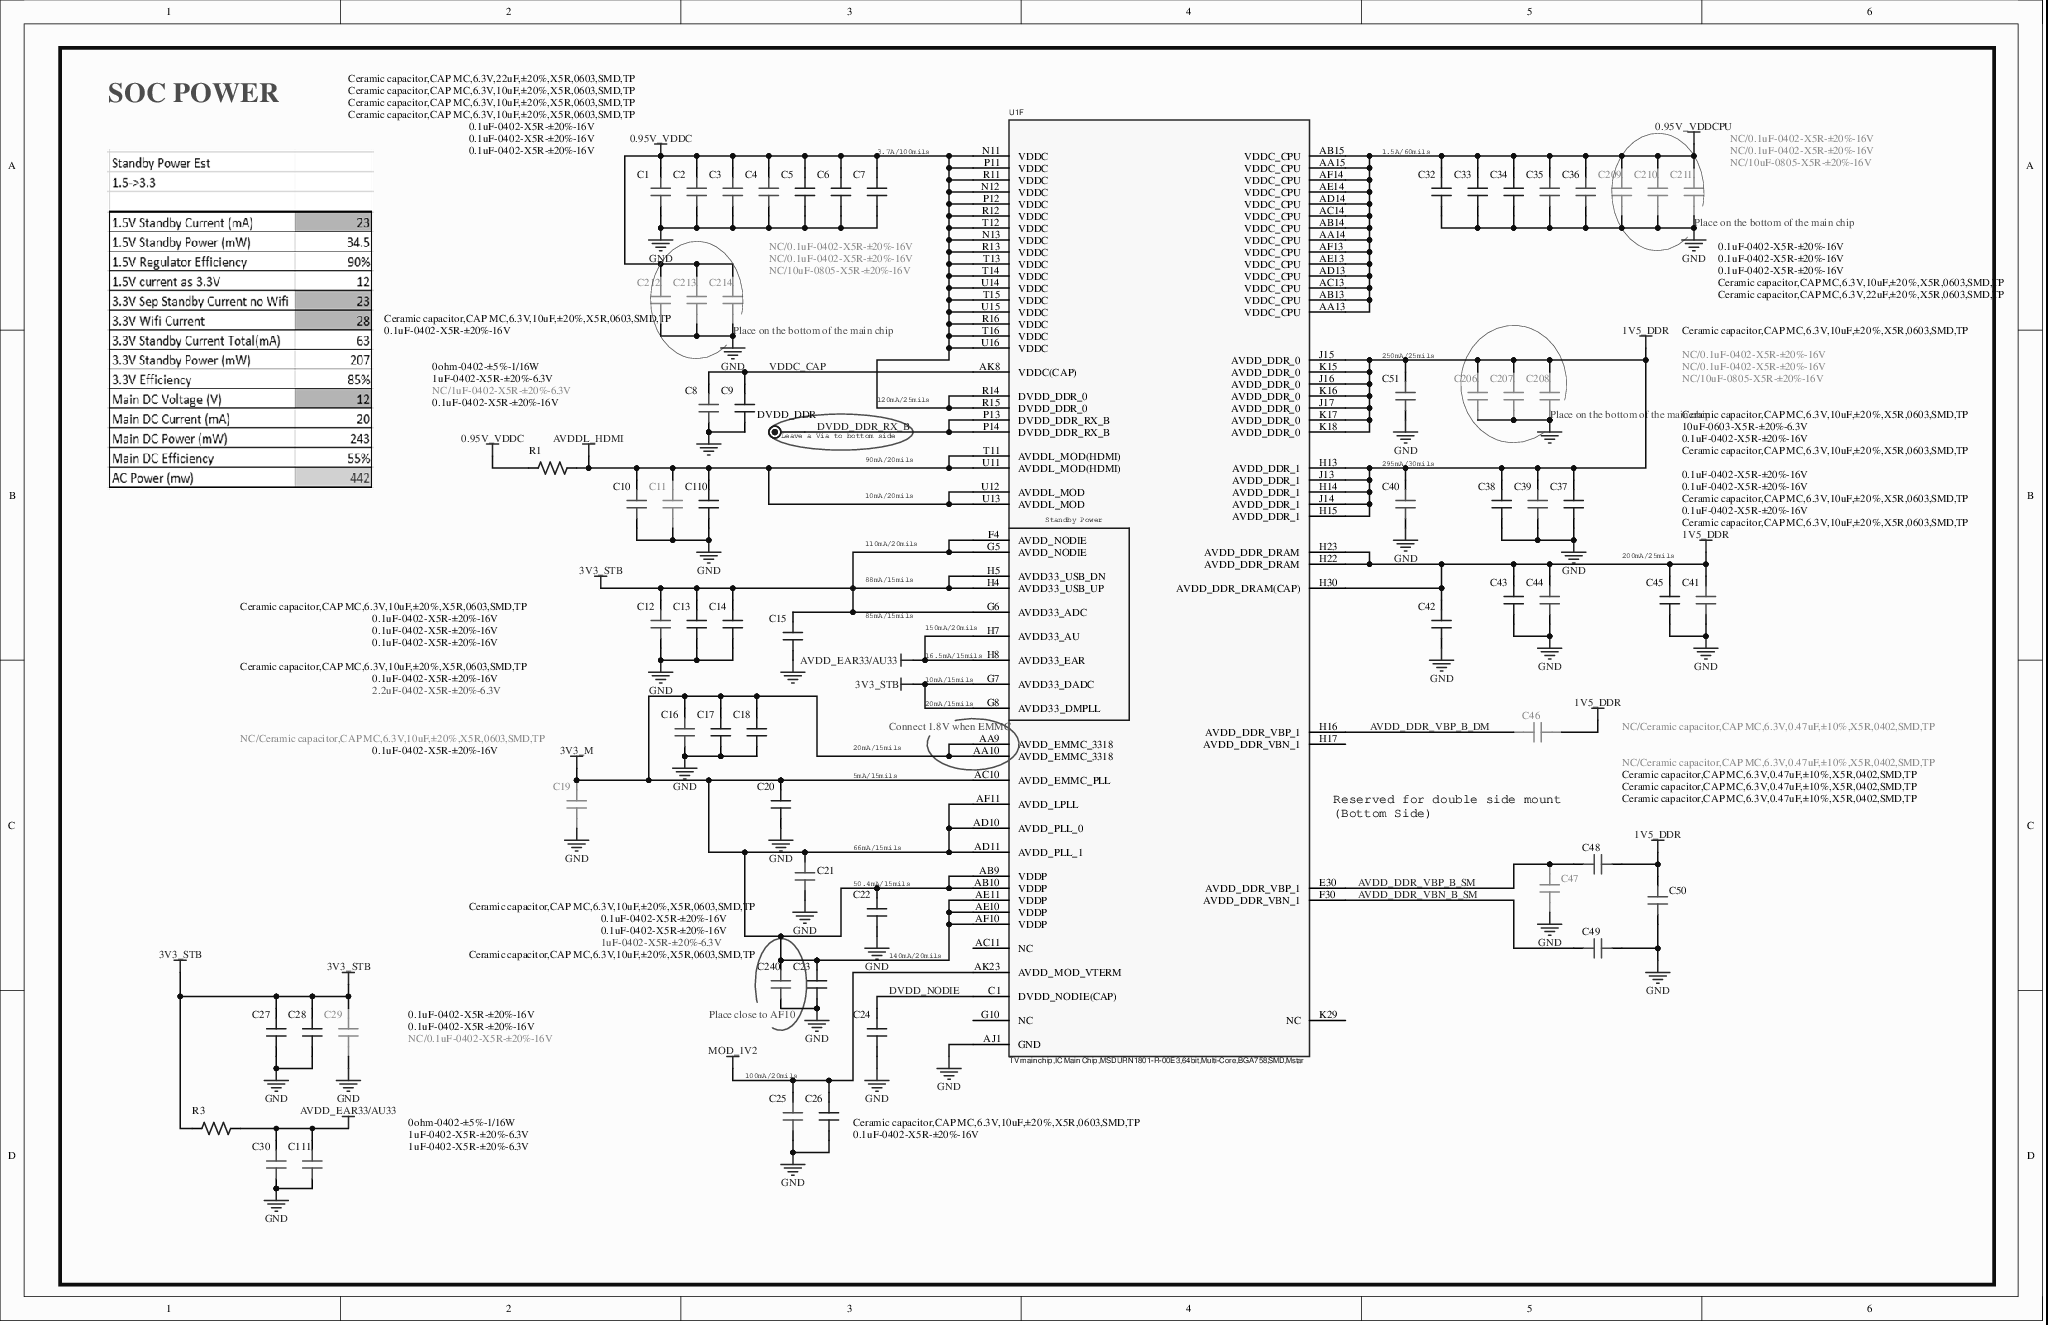
[diagram p0: MISC86290-7.SchDoc]
# Altium project MISC86290.PrjPcb (part 6 of 13)

## Sheet MISC86290-7.SchDoc
size 431 x 279 mm

### Parts
C1  Ceramic capacitor,CAP MC,6.3V,22uF,±20%,X5R,0603,SMD,TP  [C0603]
C2  Ceramic capacitor,CAP MC,6.3V,10uF,±20%,X5R,0603,SMD,TP  [C0603]
C3  Ceramic capacitor,CAP MC,6.3V,10uF,±20%,X5R,0603,SMD,TP  [C0603]
C4  Ceramic capacitor,CAP MC,6.3V,10uF,±20%,X5R,0603,SMD,TP  [C0603]
C5  0.1uF-0402-X5R-±20%-16V  [C0402]
C6  0.1uF-0402-X5R-±20%-16V  [C0402]
C7  0.1uF-0402-X5R-±20%-16V  [C0402]
C8  Ceramic capacitor,CAP MC,6.3V,10uF,±20%,X5R,0603,SMD,TP  [C0603]
C9  0.1uF-0402-X5R-±20%-16V  [C0402]
C10  1uF-0402-X5R-±20%-6.3V  [C0402]
C11  NC/1uF-0402-X5R-±20%-6.3V  [C0402]
C12  Ceramic capacitor,CAP MC,6.3V,10uF,±20%,X5R,0603,SMD,TP  [C0603]
C13  0.1uF-0402-X5R-±20%-16V  [C0402]
C14  0.1uF-0402-X5R-±20%-16V  [C0402]
C15  0.1uF-0402-X5R-±20%-16V  [C0402]
C16  Ceramic capacitor,CAP MC,6.3V,10uF,±20%,X5R,0603,SMD,TP  [C0603]
C17  0.1uF-0402-X5R-±20%-16V  [C0402]
C18  2.2uF-0402-X5R-±20%-6.3V  [C0402]
C19  NC/Ceramic capacitor,CAP MC,6.3V,10uF,±20%,X5R,0603,SMD,TP  [C0603]
C20  0.1uF-0402-X5R-±20%-16V  [C0402]
C21  Ceramic capacitor,CAP MC,6.3V,10uF,±20%,X5R,0603,SMD,TP  [C0603]
C22  0.1uF-0402-X5R-±20%-16V  [C0402]
C23  0.1uF-0402-X5R-±20%-16V  [C0402]
C24  1uF-0402-X5R-±20%-6.3V  [C0402]
C25  Ceramic capacitor,CAP MC,6.3V,10uF,±20%,X5R,0603,SMD,TP  [C0603]
C26  0.1uF-0402-X5R-±20%-16V  [C0402]
C27  0.1uF-0402-X5R-±20%-16V  [C0402]
C28  0.1uF-0402-X5R-±20%-16V  [C0402]
C29  NC/0.1uF-0402-X5R-±20%-16V  [C0402]
C30  1uF-0402-X5R-±20%-6.3V  [C0402]
C32  0.1uF-0402-X5R-±20%-16V  [C0402]
C33  0.1uF-0402-X5R-±20%-16V  [C0402]
C34  0.1uF-0402-X5R-±20%-16V  [C0402]
C35  Ceramic capacitor,CAP MC,6.3V,10uF,±20%,X5R,0603,SMD,TP  [C0603]
C36  Ceramic capacitor,CAP MC,6.3V,22uF,±20%,X5R,0603,SMD,TP  [C0603]
C37  10uF-0603-X5R-±20%-6.3V  [C0603]
C38  0.1uF-0402-X5R-±20%-16V  [C0402]
C39  Ceramic capacitor,CAP MC,6.3V,10uF,±20%,X5R,0603,SMD,TP  [C0603]
C40  Ceramic capacitor,CAP MC,6.3V,10uF,±20%,X5R,0603,SMD,TP  [C0603]
C41  Ceramic capacitor,CAP MC,6.3V,10uF,±20%,X5R,0603,SMD,TP  [C0603]
C42  0.1uF-0402-X5R-±20%-16V  [C0402]
C43  0.1uF-0402-X5R-±20%-16V  [C0402]
C44  Ceramic capacitor,CAP MC,6.3V,10uF,±20%,X5R,0603,SMD,TP  [C0603]
C45  0.1uF-0402-X5R-±20%-16V  [C0402]
C46  NC/Ceramic capacitor,CAP MC,6.3V,0.47uF,±10%,X5R,0402,SMD,TP  [C0402]
C47  NC/Ceramic capacitor,CAP MC,6.3V,0.47uF,±10%,X5R,0402,SMD,TP  [C0402]
C48  Ceramic capacitor,CAP MC,6.3V,0.47uF,±10%,X5R,0402,SMD,TP  [C0402]
C49  Ceramic capacitor,CAP MC,6.3V,0.47uF,±10%,X5R,0402,SMD,TP  [C0402]
C50  Ceramic capacitor,CAP MC,6.3V,0.47uF,±10%,X5R,0402,SMD,TP  [C0402]
C51  Ceramic capacitor,CAP MC,6.3V,10uF,±20%,X5R,0603,SMD,TP  [C0603]
C110  0.1uF-0402-X5R-±20%-16V  [C0402]
C111  1uF-0402-X5R-±20%-6.3V  [C0402]
C206  NC/0.1uF-0402-X5R-±20%-16V  [C0402]
C207  NC/0.1uF-0402-X5R-±20%-16V  [C0402]
C208  NC/10uF-0805-X5R-±20%-16V  [C0805]
C209  NC/0.1uF-0402-X5R-±20%-16V  [C0402]
C210  NC/0.1uF-0402-X5R-±20%-16V  [C0402]
C211  NC/10uF-0805-X5R-±20%-16V  [C0805]
C212  NC/0.1uF-0402-X5R-±20%-16V  [C0402]
C213  NC/0.1uF-0402-X5R-±20%-16V  [C0402]
C214  NC/10uF-0805-X5R-±20%-16V  [C0805]
C240  Ceramic capacitor,CAP MC,6.3V,10uF,±20%,X5R,0603,SMD,TP  [C0603]
DVDD_DDR  TEST  [TP-20]  (value not drawn)
R1  0ohm-0402-±5%-1/16W  [R0402]
R3  0ohm-0402-±5%-1/16W  [R0402]
U1  TV main chip,IC Main Chip,MSDURN1801-R-00E3,64bit,Multi-Core,BGA758,SMD,Mstar  [BGA758/0.65]  (part F of 7)

### Nets
0.95V_VDDC: C1.2 C2.2 C3.2 C4.2 C5.1 C6.1 C7.1 C212.1 C213.1 C214.1 R1.1 U1.N11(VDDC) U1.N12(VDDC) U1.N13(VDDC) U1.P11(VDDC) U1.P12(VDDC) U1.R11(VDDC) U1.R12(VDDC) U1.R13(VDDC) U1.R14(DVDD_DDR_0) U1.R15(DVDD_DDR_0) U1.R16(VDDC) U1.T12(VDDC) U1.T13(VDDC) U1.T14(VDDC) U1.T15(VDDC) U1.T16(VDDC) U1.U14(VDDC) U1.U15(VDDC) U1.U16(VDDC)
0.95V_VDDCPU: C32.1 C33.1 C34.1 C35.2 C36.2 C209.1 C210.1 C211.1 U1.AA13(VDDC_CPU) U1.AA14(VDDC_CPU) U1.AA15(VDDC_CPU) U1.AB13(VDDC_CPU) U1.AB14(VDDC_CPU) U1.AB15(VDDC_CPU) U1.AC13(VDDC_CPU) U1.AC14(VDDC_CPU) U1.AD13(VDDC_CPU) U1.AD14(VDDC_CPU) U1.AE13(VDDC_CPU) U1.AE14(VDDC_CPU) U1.AF13(VDDC_CPU) U1.AF14(VDDC_CPU)
1V5_DDR: C37.1 C38.1 C39.2 C40.2 C41.2 C42.1 C43.1 C44.2 C45.1 C46.2 C48.1 C50.1 C51.2 C206.1 C207.1 C208.1 U1.H13(AVDD_DDR_1) U1.H14(AVDD_DDR_1) U1.H15(AVDD_DDR_1) U1.H22(AVDD_DDR_DRAM) U1.H23(AVDD_DDR_DRAM) U1.H30(AVDD_DDR_DRAM(CAP)) U1.J13(AVDD_DDR_1) U1.J14(AVDD_DDR_1) U1.J15(AVDD_DDR_0) U1.J16(AVDD_DDR_0) U1.J17(AVDD_DDR_0) U1.K15(AVDD_DDR_0) U1.K16(AVDD_DDR_0) U1.K17(AVDD_DDR_0) U1.K18(AVDD_DDR_0)
3V3_M: C16.2 C17.1 C18.1 C19.2 C20.1 C21.2 C22.1 C23.1 C240.2 U1.AA9(AVDD_EMMC_3318) U1.AA10(AVDD_EMMC_3318) U1.AB9(VDDP) U1.AB10(VDDP) U1.AC10(AVDD_EMMC_PLL) U1.AD10(AVDD_PLL_0) U1.AD11(AVDD_PLL_1) U1.AE10(VDDP) U1.AE11(VDDP) U1.AF10(VDDP) U1.AF11(AVDD_LPLL)
3V3_STB: C12.2 C13.1 C14.1 C15.1 C27.1 C28.1 C29.1 R3.1 U1.F4(AVDD_NODIE) U1.G5(AVDD_NODIE) U1.G6(AVDD33_ADC) U1.G7(AVDD33_DADC) U1.G8(AVDD33_DMPLL) U1.H4(AVDD33_USB_UP) U1.H5(AVDD33_USB_DN)
AVDD_EAR33/AU33: C30.2 C111.2 R3.2 U1.H7(AVDD33_AU) U1.H8(AVDD33_EAR)
AVDDL_HDMI: C10.2 C11.2 C110.1 R1.2 U1.T11(AVDDL_MOD(HDMI)) U1.U11(AVDDL_MOD(HDMI)) U1.U12(AVDDL_MOD) U1.U13(AVDDL_MOD)
GND: C1.1 C2.1 C3.1 C4.1 C5.2 C6.2 C7.2 C8.1 C9.2 C10.1 C11.1 C12.1 C13.2 C14.2 C15.2 C16.1 C17.2 C18.2 C19.1 C20.2 C21.1 C22.2 C23.2 C24.2 C25.1 C26.2 C27.2 C28.2 C29.2 C30.1 C32.2 C33.2 C34.2 C35.1 C36.1 C37.2 C38.2 C39.1 C40.1 C41.1 C42.2 C43.2 C44.1 C45.2 C47.1 C49.1 C50.2 C51.1 C110.2 C111.1 C206.2 C207.2 C208.2 C209.2 C210.2 C211.2 C212.2 C213.2 C214.2 C240.1 U1.AJ1(GND)
MOD_1V2: C25.2 C26.1 U1.AK23(AVDD_MOD_VTERM)
AVDD_DDR_VBN_B_SM: C49.2 U1.F30(AVDD_DDR_VBN_1)
AVDD_DDR_VBP_B_DM: C46.1 U1.H16(AVDD_DDR_VBP_1)
AVDD_DDR_VBP_B_SM: C47.2 C48.2 U1.E30(AVDD_DDR_VBP_1)
DVDD_DDR_RX_B: DVDD_DDR.1 U1.P13(DVDD_DDR_RX_B) U1.P14(DVDD_DDR_RX_B)
DVDD_NODIE: C24.1 U1.C1(DVDD_NODIE(CAP))
VDDC_CAP: C8.2 C9.1 U1.AK8(VDDC(CAP))

Not connected (* = marked no-connect by the designer): U1 AC11(NC)* G10(NC)* H17(AVDD_DDR_VBN_1)* K29(NC)*

### Notes on the sheet
- SOC POWER
- (near C7) 3.7A/100mils
- (near C32) 1.5A/60mils
- (near C211) Place on the bottom of the main chip
- (near C214) Place on the bottom of the main chip
- (near C51) 250mA/25mils
- (near DVDD_DDR) Leave a Via to bottom side
- 120mA/25mils
- (near C208) Place on the bottom of the main chip
- 10mA/20mils
- 90mA/20mils
- (near C40) 295mA/30mils
- 110mA/20mils
- (near C45) 200mA/25mils
- 88mA/15mils
- 85mA/15mils
- (near U1) 16.5mA/15mils
- (near U1) 150mA/20mils
- (near U1) 10mA/15mils
- (near U1) Connect 1.8V when EMMC
- (near U1) 20mA/15mils
- 20mA/15mils
- 5mA/15mils
- 66mA/15mils
- Reserved for double side mount
  (Bottom Side)
- (near C22) 50.4mA/15mils
- (near C22) 140mA/20mils
- Place close to AF10
- (near C25) 100mA/20mils

### Library data of the parts
C1 C36 = 004.003.0000671-D: Ceramic capacitor,CAP MC,6.3V,22uF,±20%,X5R,0603,SMD,TP-D
C2-C4 C8 C12 C16 C19 C21 C25 C35 C39-C41 C44 C51 C240 = 004.003.0000383-D: Ceramic capacitor,CAP MC,6.3V,10uF,±20%,X5R,0603,SMD,TP-D
C5-C7 C9 C13-C15 C17 C18 C20 C22-C24 C26-C29 C32-C34 C38 C42 C43 C45 C110 C206 C207 C209 C210 C212 C213 = 0.1uF-0402-X5R-±20%-16V-D
C10 C11 C30 C111 = 004.003.0000100-D: Ceramic capacitor,CAP MC,6.3V,2.2uF,±20%,X5R,0402,SMD,TP-D
C37 = 10uF-0603-X5R-±20%-6.3V-D
C46-C50 = 004.003.0000361-D: Ceramic capacitor,CAP MC,6.3V,0.47uF,±10%,X5R,0402,SMD,TP-D
C208 C211 C214 = 10uF-0805-X5R-±20%-16V-D
R1 R3 = 0ohm-0402-±5%-1/16W-D
U1 = 004.016.0001110-D: TV main chip,IC Main Chip,MSDURN1801-Z1,64bit,Multi-Core,BGA758,SMD,Mstar-D

## Sheet MISC86290-8.SchDoc
size 381 x 241 mm
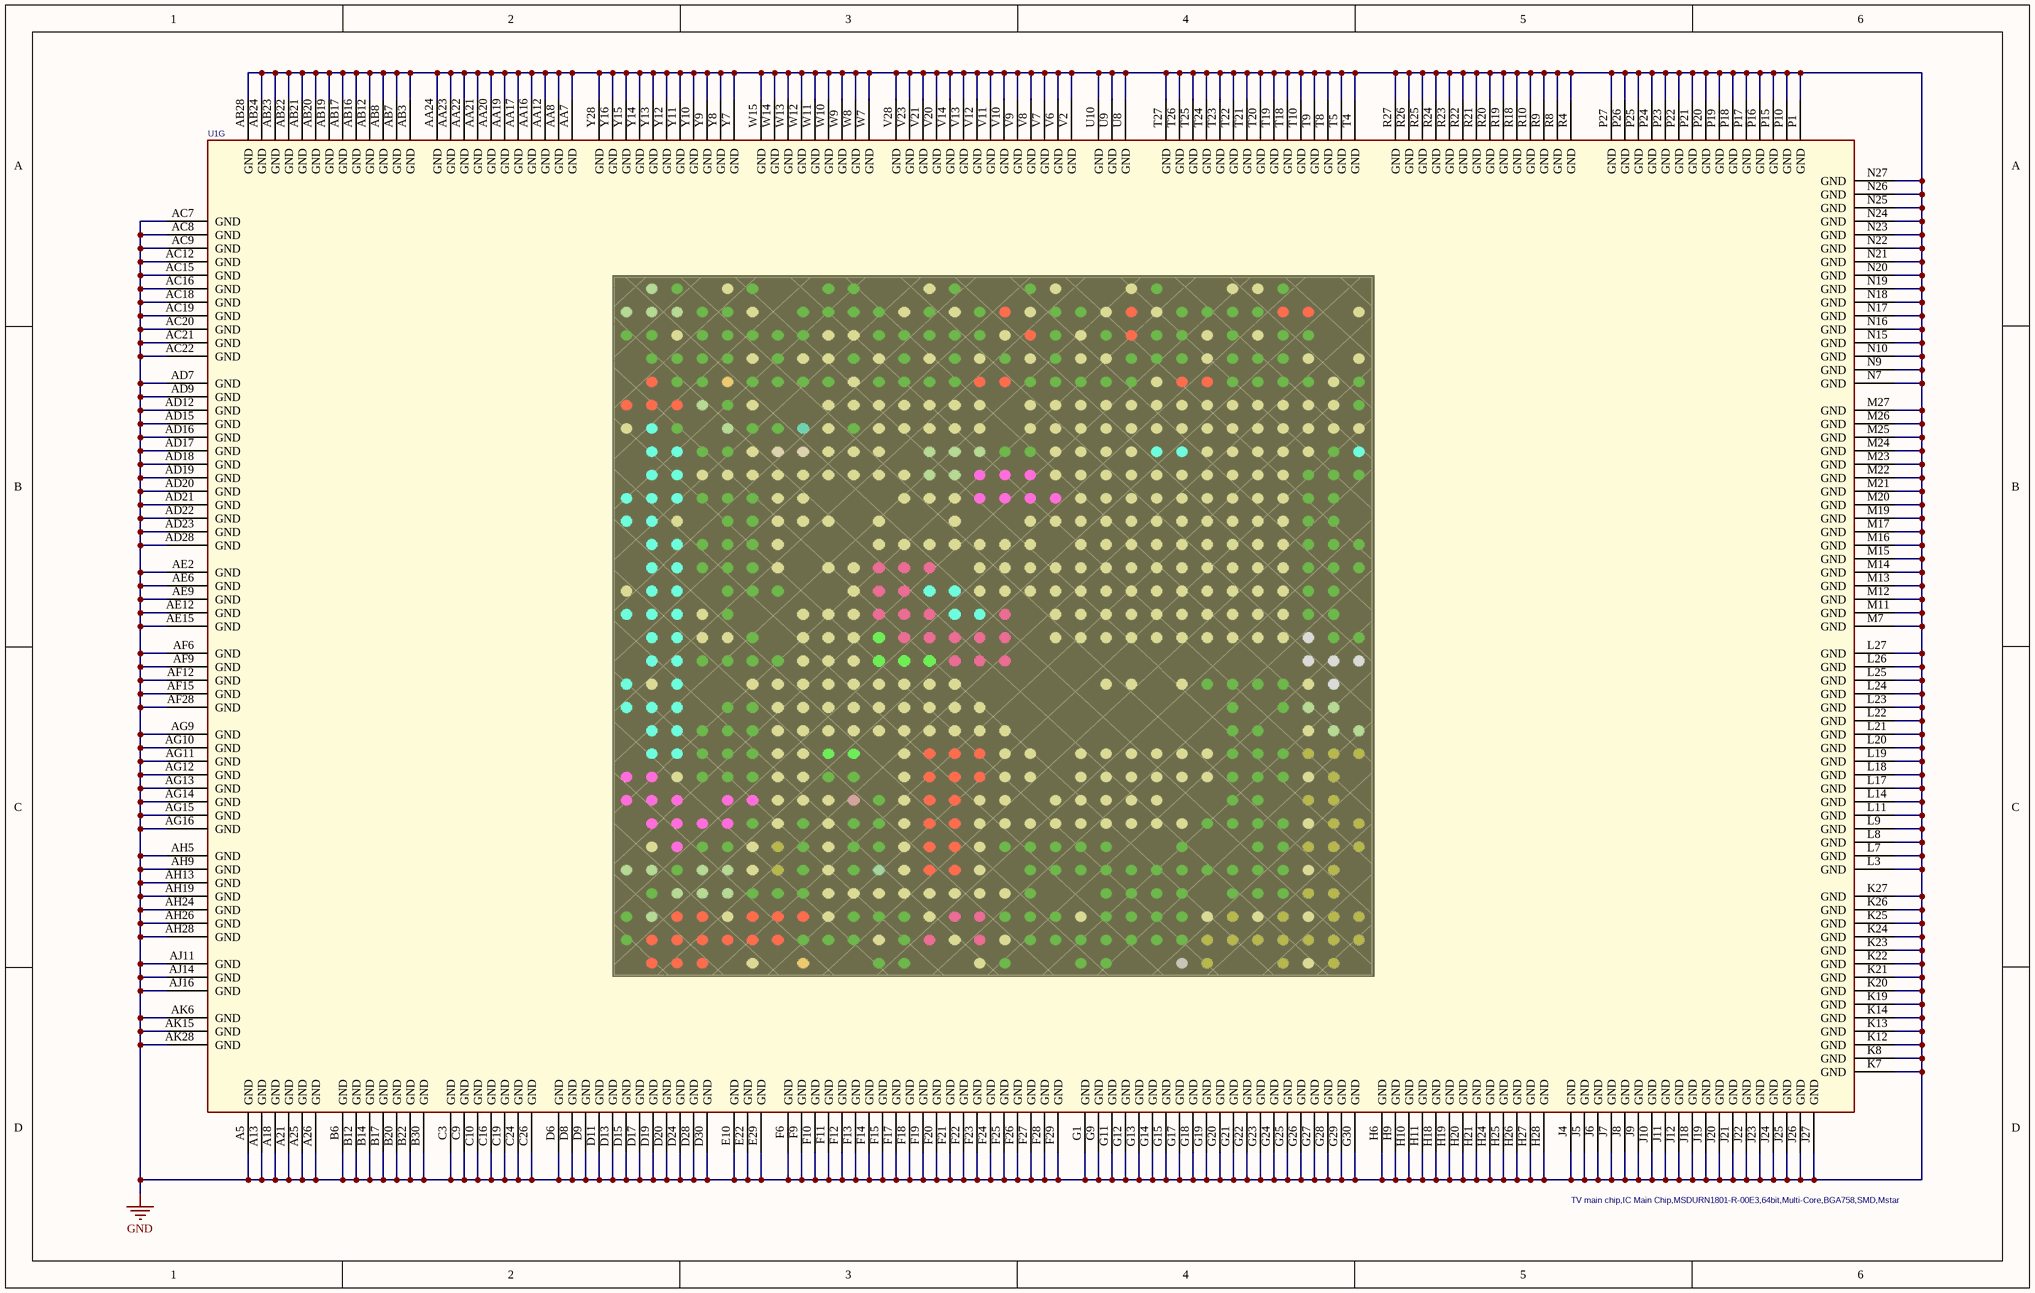
[diagram p1: MISC86290-8.SchDoc]

### Parts
U1  TV main chip,IC Main Chip,MSDURN1801-R-00E3,64bit,Multi-Core,BGA758,SMD,Mstar  [BGA758/0.65]  (part G of 7)

### Nets
GND: U1.A5(GND) U1.A13(GND) U1.A18(GND) U1.A21(GND) U1.A25(GND) U1.A26(GND) U1.AA7(GND) U1.AA8(GND) U1.AA12(GND) U1.AA16(GND) U1.AA17(GND) U1.AA19(GND) U1.AA20(GND) U1.AA21(GND) U1.AA22(GND) U1.AA23(GND) U1.AA24(GND) U1.AB3(GND) U1.AB7(GND) U1.AB8(GND) U1.AB12(GND) U1.AB16(GND) U1.AB17(GND) U1.AB19(GND) U1.AB20(GND) U1.AB21(GND) U1.AB22(GND) U1.AB23(GND) U1.AB24(GND) U1.AB28(GND) U1.AC7(GND) U1.AC8(GND) U1.AC9(GND) U1.AC12(GND) U1.AC15(GND) U1.AC16(GND) U1.AC18(GND) U1.AC19(GND) U1.AC20(GND) U1.AC21(GND) U1.AC22(GND) U1.AD7(GND) U1.AD9(GND) U1.AD12(GND) U1.AD15(GND) U1.AD16(GND) U1.AD17(GND) U1.AD18(GND) U1.AD19(GND) U1.AD20(GND) U1.AD21(GND) U1.AD22(GND) U1.AD23(GND) U1.AD28(GND) U1.AE2(GND) U1.AE6(GND) U1.AE9(GND) U1.AE12(GND) U1.AE15(GND) U1.AF6(GND) U1.AF9(GND) U1.AF12(GND) U1.AF15(GND) U1.AF28(GND) U1.AG9(GND) U1.AG10(GND) U1.AG11(GND) U1.AG12(GND) U1.AG13(GND) U1.AG14(GND) U1.AG15(GND) U1.AG16(GND) U1.AH5(GND) U1.AH9(GND) U1.AH13(GND) U1.AH19(GND) U1.AH24(GND) U1.AH26(GND) U1.AH28(GND) U1.AJ11(GND) U1.AJ14(GND) U1.AJ16(GND) U1.AK6(GND) U1.AK15(GND) U1.AK28(GND) U1.B6(GND) U1.B12(GND) U1.B14(GND) U1.B17(GND) U1.B20(GND) U1.B22(GND) U1.B30(GND) U1.C3(GND) U1.C9(GND) U1.C10(GND) U1.C16(GND) U1.C19(GND) U1.C24(GND) U1.C26(GND) U1.D6(GND) U1.D8(GND) U1.D9(GND) U1.D11(GND) U1.D13(GND) U1.D15(GND) U1.D17(GND) U1.D19(GND) U1.D20(GND) U1.D24(GND) U1.D28(GND) U1.D30(GND) U1.E10(GND) U1.E22(GND) U1.E29(GND) U1.F6(GND) U1.F9(GND) U1.F10(GND) U1.F11(GND) U1.F12(GND) U1.F13(GND) U1.F14(GND) U1.F15(GND) U1.F17(GND) U1.F18(GND) U1.F19(GND) U1.F20(GND) U1.F21(GND) U1.F22(GND) U1.F23(GND) U1.F24(GND) U1.F25(GND) U1.F26(GND) U1.F27(GND) U1.F28(GND) U1.F29(GND) U1.G1(GND) U1.G9(GND) U1.G11(GND) U1.G12(GND) U1.G13(GND) U1.G14(GND) U1.G15(GND) U1.G17(GND) U1.G18(GND) U1.G19(GND) U1.G20(GND) U1.G21(GND) U1.G22(GND) U1.G23(GND) U1.G24(GND) U1.G25(GND) U1.G26(GND) U1.G27(GND) U1.G28(GND) U1.G29(GND) U1.G30(GND) U1.H6(GND) U1.H9(GND) U1.H10(GND) U1.H11(GND) U1.H18(GND) U1.H19(GND) U1.H20(GND) U1.H21(GND) U1.H24(GND) U1.H25(GND) U1.H26(GND) U1.H27(GND) U1.H28(GND) U1.J4(GND) U1.J5(GND) U1.J6(GND) U1.J7(GND) U1.J8(GND) U1.J9(GND) U1.J10(GND) U1.J11(GND) U1.J12(GND) U1.J18(GND) U1.J19(GND) U1.J20(GND) U1.J21(GND) U1.J22(GND) U1.J23(GND) U1.J24(GND) U1.J25(GND) U1.J26(GND) U1.J27(GND) U1.K7(GND) U1.K8(GND) U1.K12(GND) U1.K13(GND) U1.K14(GND) U1.K19(GND) U1.K20(GND) U1.K21(GND) U1.K22(GND) U1.K23(GND) U1.K24(GND) U1.K25(GND) U1.K26(GND) U1.K27(GND) U1.L3(GND) U1.L7(GND) U1.L8(GND) U1.L9(GND) U1.L11(GND) U1.L14(GND) U1.L17(GND) U1.L18(GND) U1.L19(GND) U1.L20(GND) U1.L21(GND) U1.L22(GND) U1.L23(GND) U1.L24(GND) U1.L25(GND) U1.L26(GND) U1.L27(GND) U1.M7(GND) U1.M11(GND) U1.M12(GND) U1.M13(GND) U1.M14(GND) U1.M15(GND) U1.M16(GND) U1.M17(GND) U1.M19(GND) U1.M20(GND) U1.M21(GND) U1.M22(GND) U1.M23(GND) U1.M24(GND) U1.M25(GND) U1.M26(GND) U1.M27(GND) U1.N7(GND) U1.N9(GND) U1.N10(GND) U1.N15(GND) U1.N16(GND) U1.N17(GND) U1.N18(GND) U1.N19(GND) U1.N20(GND) U1.N21(GND) U1.N22(GND) U1.N23(GND) U1.N24(GND) U1.N25(GND) U1.N26(GND) U1.N27(GND) U1.P1(GND) U1.P10(GND) U1.P15(GND) U1.P16(GND) U1.P17(GND) U1.P18(GND) U1.P19(GND) U1.P20(GND) U1.P21(GND) U1.P22(GND) U1.P23(GND) U1.P24(GND) U1.P25(GND) U1.P26(GND) U1.P27(GND) U1.R4(GND) U1.R8(GND) U1.R9(GND) U1.R10(GND) U1.R18(GND) U1.R19(GND) U1.R20(GND) U1.R21(GND) U1.R22(GND) U1.R23(GND) U1.R24(GND) U1.R25(GND) U1.R26(GND) U1.R27(GND) U1.T4(GND) U1.T5(GND) U1.T8(GND) U1.T9(GND) U1.T10(GND) U1.T18(GND) U1.T19(GND) U1.T20(GND) U1.T21(GND) U1.T22(GND) U1.T23(GND) U1.T24(GND) U1.T25(GND) U1.T26(GND) U1.T27(GND) U1.U8(GND) U1.U9(GND) U1.U10(GND) U1.V2(GND) U1.V6(GND) U1.V7(GND) U1.V8(GND) U1.V9(GND) U1.V10(GND) U1.V11(GND) U1.V12(GND) U1.V13(GND) U1.V14(GND) U1.V20(GND) U1.V21(GND) U1.V23(GND) U1.V28(GND) U1.W7(GND) U1.W8(GND) U1.W9(GND) U1.W10(GND) U1.W11(GND) U1.W12(GND) U1.W13(GND) U1.W14(GND) U1.W15(GND) U1.Y7(GND) U1.Y8(GND) U1.Y9(GND) U1.Y10(GND) U1.Y11(GND) U1.Y12(GND) U1.Y13(GND) U1.Y14(GND) U1.Y15(GND) U1.Y16(GND) U1.Y28(GND)

### Library data of the parts
U1 = 004.016.0001110-D: as U1 on sheet MISC86290-7